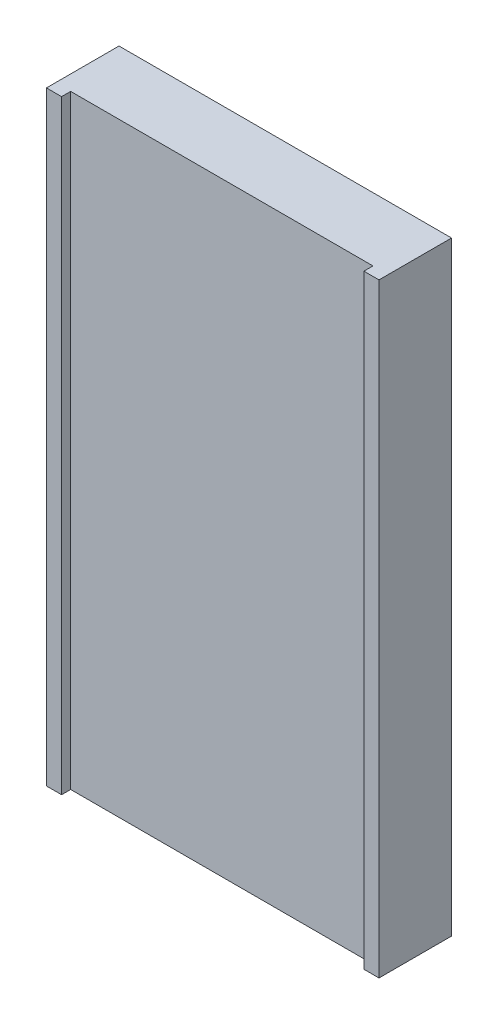
SolidWorks part; units mm, degrees
ref_plane "前视基准面" through (0, 0, 0) normal (0, 0, 1) x (1, 0, 0)
ref_plane "上视基准面" through (0, 0, 0) normal (0, 1, 0) x (1, 0, 0)
ref_plane "右视基准面" through (0, 0, 0) normal (1, 0, 0) x (0, 0, -1)
sketch "草图1" plane through (0, 0, 0) normal (0, 0, 1) x (1, 0, 0)
  line L1 (-27.5, -50) -> (27.5, -50)
  line L2 (-27.5, -50) -> (-27.5, 50)
  line L3 (-27.5, 50) -> (27.5, 50)
  line L4 (27.5, -50) -> (27.5, 50)
  line L5 (-27.5, -50) -> (27.5, 50) construction
  line L6 (-27.5, 50) -> (27.5, -50) construction
  point P0 (0, 0)
  dimension "D1" = 55
  dimension "D2" = 100
extrude "凸台-拉伸1" add sketch "草图1" along normal blind 12
sketch "草图2" plane through (0, 0, 12) normal (0, 0, 1) x (1, 0, 0)
  line L0 (27.5, 50) -> (-27.5, 50) construction
  line L1 (-25, -50) -> (25, -50)
  line L2 (-25, -50) -> (-25, 50)
  line L3 (-25, 50) -> (25, 50)
  line L4 (25, -50) -> (25, 50)
  line L5 (-25, -50) -> (25, 50) construction
  line L6 (-25, 50) -> (25, -50) construction
  point P0 (0, 0)
  dimension "D1" = 50
extrude "切除-拉伸1" cut sketch "草图2" against normal blind 1.5
